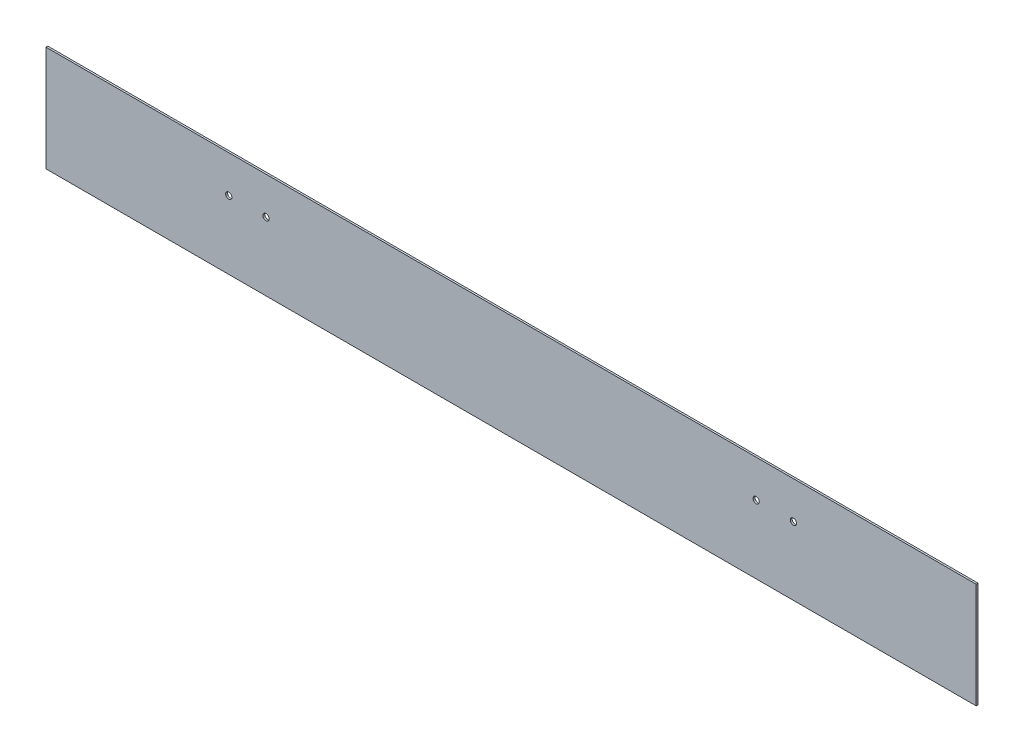
SolidWorks part; units mm, degrees
material "1060 合金"
ref_plane "前视基准面" through (0, 0, 0) normal (0, 0, 1) x (1, 0, 0)
ref_plane "上视基准面" through (0, 0, 0) normal (0, 1, 0) x (1, 0, 0)
ref_plane "右视基准面" through (0, 0, 0) normal (1, 0, 0) x (0, 0, -1)
sketch "草图1" plane through (0, 0, 0) normal (0, 0, 1) x (1, 0, 0)
  line L1 (-750, -80) -> (750, -80)
  line L2 (-750, -80) -> (-750, 80)
  line L3 (-750, 80) -> (750, 80)
  line L4 (750, -80) -> (750, 80)
  line L5 (-750, -80) -> (750, 80) construction
  line L6 (-750, 80) -> (750, -80) construction
  point P0 (0, 0)
  dimension "D1" = 1500
  dimension "D2" = 160
extrude "凸台-拉伸1" add sketch "草图1" along normal blind 3
sketch "草图3" plane through (0, 0, 3) normal (0, 0, 1) x (1, 0, 0)
  circle A0 centre (-455.26, 30) radius 5
  circle A1 centre (-395.26, 30) radius 5
  dimension "D3" = 10
  dimension "D1" = 60
extrude "切除-拉伸1" cut sketch "草图3" against normal through all both
mirror "镜向1" about plane through (0, 0, 0) normal (1, 0, 0) of "切除-拉伸1"
sketch "草图7" plane through (0, 80, 0) normal (0, 1, 0) x (1, 0, 0)
  line L4 (750, 0) -> (-750, 0)
  line L5 (-750, 0) -> (-750, -3)
  line L6 (-750, -3) -> (750, -3)
  line L7 (750, -3) -> (750, 0)
  line L8 (750, 0) -> (-750, 0)
  line L9 (-750, 0) -> (-750, -3)
  line L10 (-750, -3) -> (750, -3)
  line L11 (750, -3) -> (750, 0)
  dimension "D1" = 0
extrude "凸台-拉伸2" add sketch "草图7" along normal blind 10
